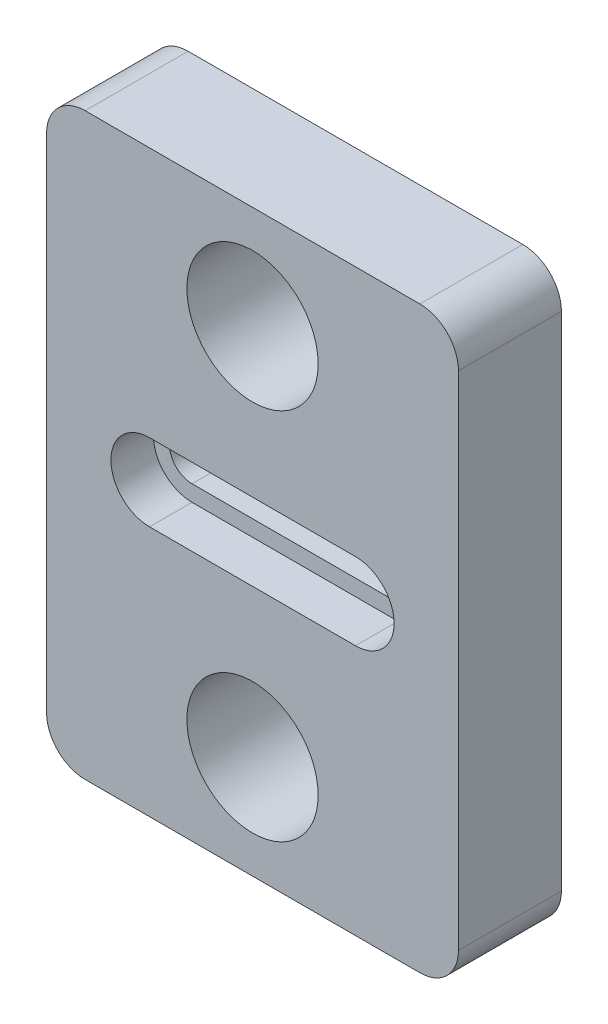
SolidWorks part; units mm, degrees
ref_plane "Front Plane" through (0, 0, 0) normal (0, 0, 1) x (1, 0, 0)
ref_plane "Top Plane" through (0, 0, 0) normal (0, 1, 0) x (1, 0, 0)
ref_plane "Right Plane" through (0, 0, 0) normal (1, 0, 0) x (0, 0, -1)
sketch "Sketch1" plane through (0, 0, 0) normal (0, 0, 1) x (1, 0, 0)
  line L1 (16, -22.5) -> (-16, -22.5)
  line L2 (16, -22.5) -> (16, 22.5)
  line L3 (16, 22.5) -> (-16, 22.5)
  line L4 (-16, -22.5) -> (-16, 22.5)
  line L5 (16, -22.5) -> (-16, 22.5) construction
  line L6 (16, 22.5) -> (-16, -22.5) construction
  point P0 (0, 0)
  dimension "D1" = 32
  dimension "D2" = 45
extrude "Boss-Extrude1" add sketch "Sketch1" along normal blind 8
hole_wizard "M12 Tapped Hole1" positions "Sketch2" profile "Sketch3" tap size "M12" standard "GB"
sketch "Sketch2" plane through (0, 0, 8) normal (0, 0, 1) x (1, 0, 0)
  point P0 (0, 0)
sketch "Sketch3" plane through (0, 0, 8) normal (1, 0, 0) x (0, -1, 0)
  line L0 (0, 0) -> (0, 8)
  line L1 (0, 8) -> (5.1, 8)
  line L2 (5.1, 8) -> (5.1, 0)
  line L5 (5.1, 0) -> (0, 0)
  line L11 (0, -6.35) -> (0, 107.95) construction
  dimension "通孔螺纹孔钻头直径" = 10.2
  dimension "通孔螺纹孔钻头深度" = 8
cosmetic thread "Cosmetic Thread1" [suppressed] parameters "D2"=12
sketch "Sketch5" plane through (0, 0, 8) normal (0, 0, 1) x (1, 0, 0)
  line L0 (-8, 0) -> (8, 0) construction
  line L1 (-8, 1.75) -> (8, 1.75)
  line L2 (-8, -1.75) -> (8, -1.75)
  arc A0 (-8, 1.75) -> (-8, -1.75) centre (-8, 0) ccw
  arc A1 (8, -1.75) -> (8, 1.75) centre (8, 0) ccw
  point P2 (0, 0)
  dimension "D5" = 1.75
  dimension "D3" = 16
extrude "Cut-Extrude1" cut sketch "Sketch5" against normal through all
sketch "Sketch6" plane through (0, 0, 8) normal (0, 0, 1) x (1, 0, 0)
  line L0 (-8, 0) -> (8, 0) construction
  line L1 (-8, 3) -> (8, 3)
  line L2 (-8, -3) -> (8, -3)
  arc A0 (-8, 3) -> (-8, -3) centre (-8, 0) ccw
  arc A1 (8, -3) -> (8, 3) centre (8, 0) ccw
  point P4 (0, 0)
  dimension "D2" = 3
  dimension "D1" = 16
extrude "Cut-Extrude2" cut sketch "Sketch6" against normal blind 3.3
fillet "Fillet1" radius 3 4 edges at (-16, 22.5, 4) (16, 22.5, 4) (16, -22.5, 4) (-16, -22.5, 4)
hole_wizard "M12 Tapped Hole2" positions "Sketch7" profile "Sketch8" tap size "M12" standard "GB" end condition through all
sketch "Sketch7" plane through (0, 0, 8) normal (0, 0, 1) x (1, 0, 0)
  point P0 (0, -14.5)
  point P2 (0, 14.5)
  dimension "D1" = 14.5
  dimension "D2" = 29
sketch "Sketch8" plane through (0, -14.5, 8) normal (1, 0, 0) x (0, -1, 0)
  line L0 (0, 0) -> (0, 8)
  line L1 (0, 8) -> (5.1, 8)
  line L2 (5.1, 8) -> (5.1, 0)
  line L5 (5.1, 0) -> (0, 0)
  line L11 (0, -6.35) -> (0, 107.95) construction
  dimension "通孔螺纹孔钻头直径" = 10.2
  dimension "通孔螺纹孔钻头深度" = 8
cosmetic thread "Cosmetic Thread2" parameters "D2"=12
cosmetic thread "Cosmetic Thread3" parameters "D2"=12
